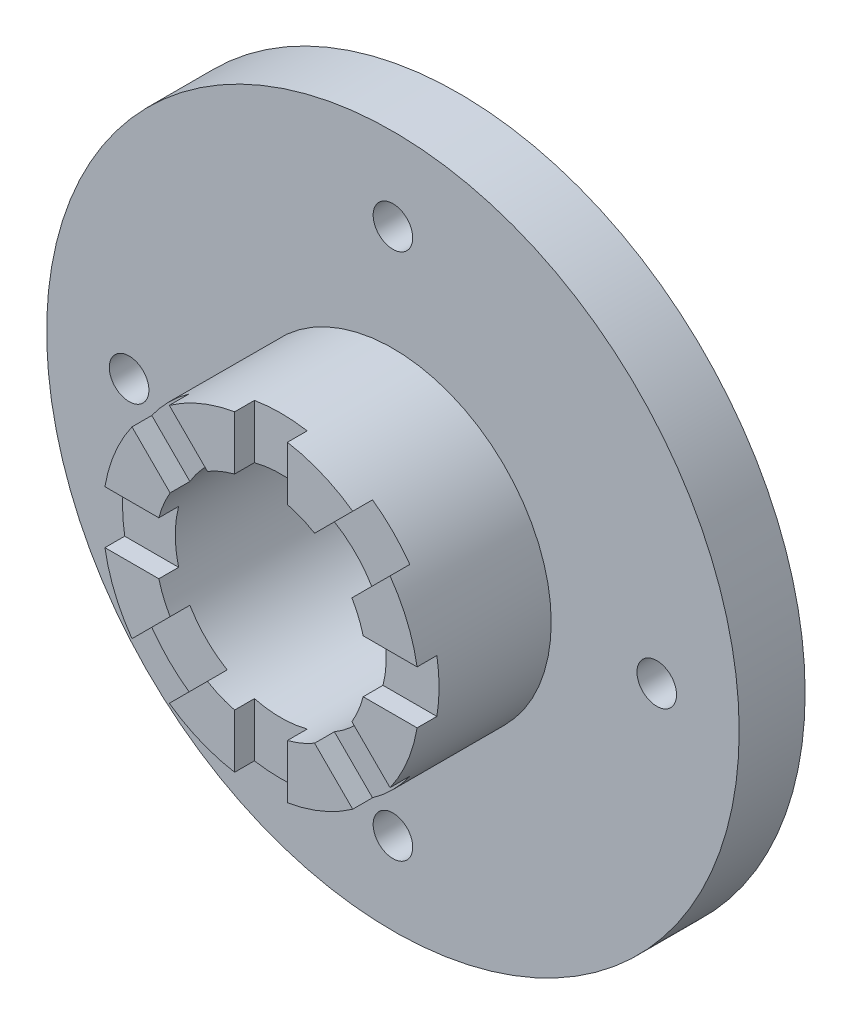
from build123d import *

# Parameters (mm, degrees)
SKETCH_1_R          = 52.5
SKETCH_1_R_2        = 16
SKETCH_1_R_3        = 3
EXTRUDE_1_DEPTH     = 10
SKETCH_2_R          = 24
SKETCH_2_R_2        = 16
EXTRUDE_2_DEPTH     = 20
CUT_EXTRUDE_START   = -3
CUT_EXTRUDE_2_DEPTH = 3


with BuildPart() as part:
    # 草图1 → 凸台-拉伸1 (new body)
    with BuildSketch(Plane.XY):
        Circle(SKETCH_1_R)
        Circle(SKETCH_1_R_2, mode=Mode.SUBTRACT)
        with Locations((0, 40)):
            Circle(SKETCH_1_R_3, mode=Mode.SUBTRACT)
        with Locations((40, 0)):
            Circle(SKETCH_1_R_3, mode=Mode.SUBTRACT)
        with Locations((0, -40)):
            Circle(SKETCH_1_R_3, mode=Mode.SUBTRACT)
        with Locations((-40, 0)):
            Circle(SKETCH_1_R_3, mode=Mode.SUBTRACT)
    extrude(amount=EXTRUDE_1_DEPTH)

    # 草图2 → 凸台-拉伸2 (add)
    with BuildSketch(Plane.XY.offset(10)):
        Circle(SKETCH_2_R)
        Circle(SKETCH_2_R_2, mode=Mode.SUBTRACT)
    extrude(amount=EXTRUDE_2_DEPTH)

    # 草图3 → 切除-拉伸2 (cut)
    with BuildSketch(Plane.XY.offset(30).offset(CUT_EXTRUDE_START)):
        with BuildLine():
            Line((-4, 23.664319132), (-4, 15.491933385))
            ThreePointArc((-4, 15.491933385), (0, 16), (4, 15.491933385))
            Line((4, 15.491933385), (4, 23.664319132))
            ThreePointArc((4, 23.664319132), (0, 24), (-4, 23.664319132))
        make_face()
        with BuildLine():
            Line((13.904773406, 19.561627655), (8.126024025, 13.782878275))
            ThreePointArc((8.126024025, 13.782878275), (11.313708499, 11.313708499), (13.782878275, 8.126024025))
            Line((13.782878275, 8.126024025), (19.561627655, 13.904773406))
            ThreePointArc((19.561627655, 13.904773406), (16.970562748, 16.970562748), (13.904773406, 19.561627655))
        make_face()
        with BuildLine():
            Line((23.664319132, 4), (15.491933385, 4))
            ThreePointArc((15.491933385, 4), (16, 0), (15.491933385, -4))
            Line((15.491933385, -4), (23.664319132, -4))
            ThreePointArc((23.664319132, -4), (24, 0), (23.664319132, 4))
        make_face()
        with BuildLine():
            Line((19.561627655, -13.904773406), (13.782878275, -8.126024025))
            ThreePointArc((13.782878275, -8.126024025), (11.313708499, -11.313708499), (8.126024025, -13.782878275))
            Line((8.126024025, -13.782878275), (13.904773406, -19.561627655))
            ThreePointArc((13.904773406, -19.561627655), (16.970562748, -16.970562748), (19.561627655, -13.904773406))
        make_face()
        with BuildLine():
            Line((4, -23.664319132), (4, -15.491933385))
            ThreePointArc((4, -15.491933385), (0, -16), (-4, -15.491933385))
            Line((-4, -15.491933385), (-4, -23.664319132))
            ThreePointArc((-4, -23.664319132), (0, -24), (4, -23.664319132))
        make_face()
        with BuildLine():
            Line((-13.904773406, -19.561627655), (-8.126024025, -13.782878275))
            ThreePointArc((-8.126024025, -13.782878275), (-11.313708499, -11.313708499), (-13.782878275, -8.126024025))
            Line((-13.782878275, -8.126024025), (-19.561627655, -13.904773406))
            ThreePointArc((-19.561627655, -13.904773406), (-16.970562748, -16.970562748), (-13.904773406, -19.561627655))
        make_face()
        with BuildLine():
            Line((-23.664319132, -4), (-15.491933385, -4))
            ThreePointArc((-15.491933385, -4), (-16, 0), (-15.491933385, 4))
            Line((-15.491933385, 4), (-23.664319132, 4))
            ThreePointArc((-23.664319132, 4), (-24, 0), (-23.664319132, -4))
        make_face()
        with BuildLine():
            Line((-19.561627655, 13.904773406), (-13.782878275, 8.126024025))
            ThreePointArc((-13.782878275, 8.126024025), (-11.313708499, 11.313708499), (-8.126024025, 13.782878275))
            Line((-8.126024025, 13.782878275), (-13.904773406, 19.561627655))
            ThreePointArc((-13.904773406, 19.561627655), (-16.970562748, 16.970562748), (-19.561627655, 13.904773406))
        make_face()
    extrude(amount=CUT_EXTRUDE_2_DEPTH, mode=Mode.SUBTRACT)


solid = part.part
